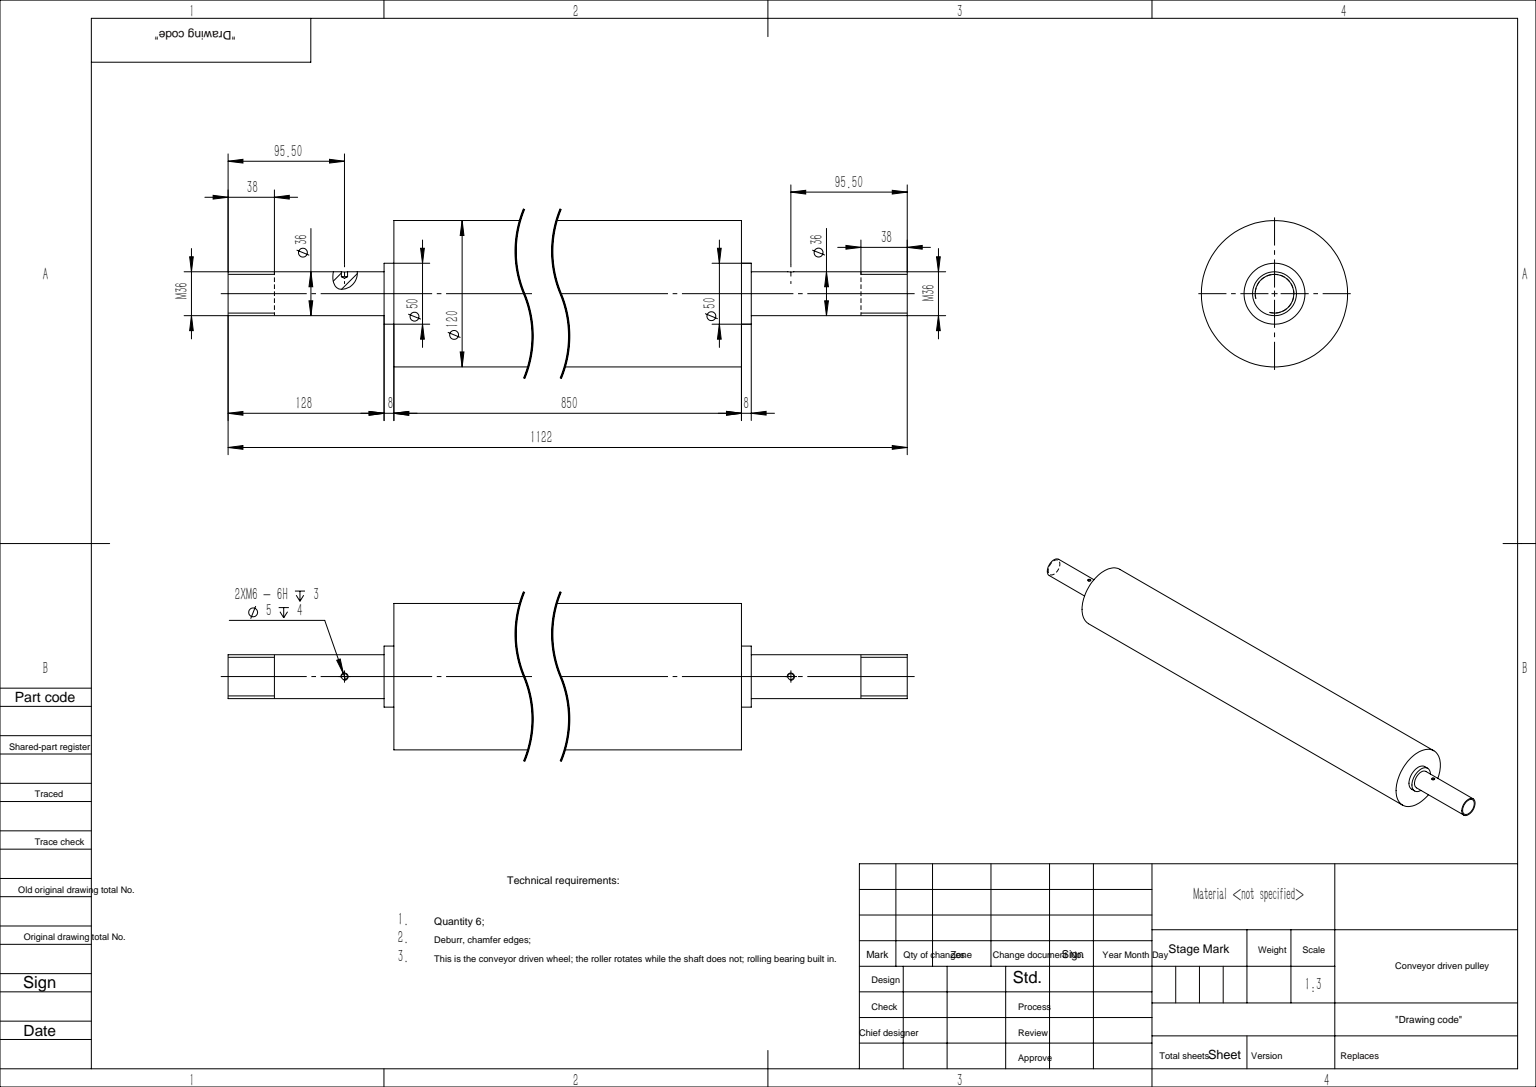
from build123d import *


with BuildPart() as part:
    # 草图1 → 旋转1 (revolve)
    with BuildSketch(Plane.XY, mode=Mode.PRIVATE) as revolve_1_sk:
        Polygon((-425, 60), (425, 60), (425, 25), (433, 25), (433, 18), (561, 18), (561, 0), (-561, 0), (-561, 18), (-433, 18), (-433, 25), (-425, 25), align=None)
    revolve(revolve_1_sk.sketch.rotate(Axis((0, 0, 0), (1, 0, 0)), 90), axis=Axis((0, 0, 0), (1, 0, 0)))

    # 草图2 → M6 螺纹孔1 (revolve, cut)
    with BuildSketch(Plane(origin=(465.5, 18, 0), x_dir=(0, 0, 1), z_dir=(1, 0, 0))):
        Polygon((0, 0), (0, 5.443375673), (2.5, 4), (2.5, 0), align=None)
    hole_wizard_m6_1 = revolve(axis=Axis((465.5, 24.35, 0), (0, -1, 0)), mode=Mode.SUBTRACT)

    # 镜向1: M6 螺纹孔1 across plane
    add(hole_wizard_m6_1.mirror(Plane(origin=(0, 0, 0), x_dir=(0, 0, 1), z_dir=(1, 0, 0))), mode=Mode.SUBTRACT)


solid = part.part
